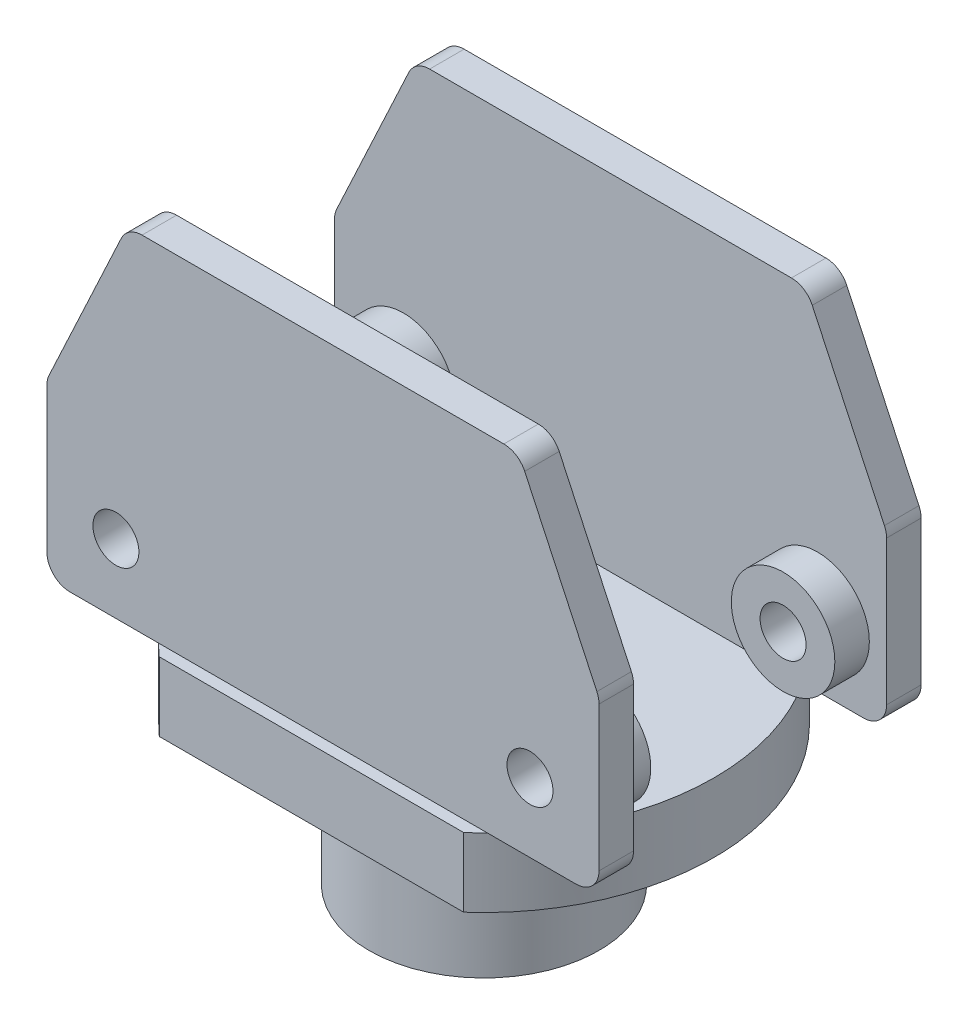
from build123d import *

# Parameters (mm, degrees)
SKETCH1_R             = 50
BOSS_EXTRUDE1_DEPTH   = 60
SKETCH2_R             = 100
BOSS_EXTRUDE2_DEPTH   = 30
CUT_EXTRUDE1_DEPTH    = 154.622914957
SKETCH4_W             = 300
SKETCH4_H             = 15
BOSS_EXTRUDE3_DEPTH   = 150
SKETCH5_W             = 30
SKETCH5_H             = 150
CUT_EXTRUDE2_DEPTH    = 319.001572323
FILLET1_R             = 10
SKETCH6_R             = 25
CUT_EXTRUDE3_DEPTH    = 150
SKETCH7_R             = 10
CUT_EXTRUDE4_DEPTH    = 306
SKETCH8_R             = 22.5
SKETCH8_R_2           = 10
BOSS_EXTRUDE4_DEPTH   = 15
BOSS_EXTRUDE4_2_DEPTH = 15
SKETCH9_R             = 22.5
SKETCH9_R_2           = 10
BOSS_EXTRUDE5_DEPTH   = 15
BOSS_EXTRUDE5_2_DEPTH = 15
CUT_EXTRUDE5_DEPTH    = 306
FILLET2_R             = 10


with BuildPart() as part:
    # Sketch1 → Boss-Extrude1 (new body)
    with BuildSketch(Plane(origin=(0, 0, 0), x_dir=(1, 0, 0), z_dir=(0, 1, 0))):
        with Locations(Location((0, 0, 0), (0, 0, 270))):
            Circle(SKETCH1_R)
    extrude(amount=BOSS_EXTRUDE1_DEPTH)

    # Sketch2 → Boss-Extrude2 (add)
    with BuildSketch(Plane(origin=(0, 60, 0), x_dir=(1, 0, 0), z_dir=(0, 1, 0))):
        with Locations(Location((0, 0, 0), (0, 0, 270))):
            Circle(SKETCH2_R)
    extrude(amount=BOSS_EXTRUDE2_DEPTH)

    # Sketch3 → Cut-Extrude1 (cut, through all)
    with BuildSketch(Plane.XZ.offset(-60)):
        Polygon((191.018311805, 75), (5.81663556, 170.543754632), (-191.018311805, 75), align=None)
        Polygon((-191.018311805, -75), (191.018311805, -75), (12.796598233, -157.049160132), align=None)
    extrude(amount=-CUT_EXTRUDE1_DEPTH, mode=Mode.SUBTRACT)

    # Sketch4 → Boss-Extrude3 (add)
    with BuildSketch(Plane(origin=(0, 90, 0), x_dir=(1, 0, 0), z_dir=(0, 1, 0))):
        with Locations((0, 62.5)):
            Rectangle(SKETCH4_W, SKETCH4_H)
        with Locations((0, -62.5)):
            Rectangle(SKETCH4_W, SKETCH4_H)
    extrude(amount=BOSS_EXTRUDE3_DEPTH)

    # Sketch5 → Cut-Extrude2 (cut, through all)
    with BuildSketch(Plane(origin=(0, 0, -70), x_dir=(-1, 0, 0), z_dir=(0, 0, -1))):
        with Locations((-135, 165)):
            Rectangle(SKETCH5_W, SKETCH5_H)
        with Locations((135, 165)):
            Rectangle(SKETCH5_W, SKETCH5_H)
    extrude(amount=-CUT_EXTRUDE2_DEPTH, mode=Mode.SUBTRACT)

    # Fillet1
    fillet1_edges = [part.edges().sort_by_distance(p)[0] for p in [
        (-120, 240, -62.5),
        (-120, 240, 62.5),
        (-120, 90, -62.5),
        (-120, 90, 62.5),
        (120, 240, 62.5),
        (120, 90, -62.5),
        (120, 90, 62.5),
        (120, 240, -62.5),
    ]]
    fillet(fillet1_edges, radius=FILLET1_R)

    # Sketch6 → Cut-Extrude3 (cut)
    with BuildSketch(Plane(origin=(0, 90, 0), x_dir=(1, 0, 0), z_dir=(0, 1, 0))):
        with Locations(Location((0, 0, 0), (0, 0, 270))):
            Circle(SKETCH6_R)
    extrude(amount=-CUT_EXTRUDE3_DEPTH, mode=Mode.SUBTRACT)

    # Sketch7 → Cut-Extrude4 (cut, through all)
    with BuildSketch(Plane(origin=(0, 0, -70), x_dir=(-1, 0, 0), z_dir=(0, 0, -1))):
        with Locations((-90, 120)):
            Circle(SKETCH7_R)
        with Locations((90, 120)):
            Circle(SKETCH7_R)
    extrude(amount=-CUT_EXTRUDE4_DEPTH, mode=Mode.SUBTRACT)

    # Sketch10 → Cut-Extrude5 (cut, through all)
    with BuildSketch(Plane(origin=(0, 0, -70), x_dir=(-1, 0, 0), z_dir=(0, 0, -1))):
        Polygon((-120, 165), (-85, 240), (-120, 240), align=None)
        Polygon((120, 165), (85, 240), (120, 240), align=None)
    extrude(amount=-CUT_EXTRUDE5_DEPTH, mode=Mode.SUBTRACT)

    # Fillet2
    fillet2_edges = [part.edges().sort_by_distance(p)[0] for p in [
        (85, 240, -62.5),
        (85, 240, 62.5),
        (120, 165, 62.5),
        (120, 165, -62.5),
        (-120, 165, -62.5),
        (-120, 165, 62.5),
        (-85, 240, 62.5),
        (-85, 240, -62.5),
    ]]
    fillet(fillet2_edges, radius=FILLET2_R)


with BuildPart() as body_2:
    # Sketch8 → Boss-Extrude4 (new body)
    with BuildSketch(Plane(origin=(0, 0, 55), x_dir=(-1, 0, 0), z_dir=(0, 0, -1))):
        with Locations((90, 120)):
            Circle(SKETCH8_R)
        with Locations((90, 120)):
            Circle(SKETCH8_R_2, mode=Mode.SUBTRACT)
    extrude(amount=BOSS_EXTRUDE4_DEPTH)


with BuildPart() as body_3:
    # Sketch8 → Boss-Extrude4 2 (new body)
    with BuildSketch(Plane(origin=(0, 0, 55), x_dir=(-1, 0, 0), z_dir=(0, 0, -1))):
        with Locations((-90, 120)):
            Circle(SKETCH8_R)
        with Locations((-90, 120)):
            Circle(SKETCH8_R_2, mode=Mode.SUBTRACT)
    extrude(amount=BOSS_EXTRUDE4_2_DEPTH)


with BuildPart() as body_4:
    # Sketch9 → Boss-Extrude5 (new body)
    with BuildSketch(Plane.XY.offset(-55)):
        with Locations((90, 120)):
            Circle(SKETCH9_R)
        with Locations((90, 120)):
            Circle(SKETCH9_R_2, mode=Mode.SUBTRACT)
    extrude(amount=BOSS_EXTRUDE5_DEPTH)


with BuildPart() as body_5:
    # Sketch9 → Boss-Extrude5 2 (new body)
    with BuildSketch(Plane.XY.offset(-55)):
        with Locations((-90, 120)):
            Circle(SKETCH9_R)
        with Locations((-90, 120)):
            Circle(SKETCH9_R_2, mode=Mode.SUBTRACT)
    extrude(amount=BOSS_EXTRUDE5_2_DEPTH)


solid = Compound([part.part, body_2.part, body_3.part, body_4.part, body_5.part])
